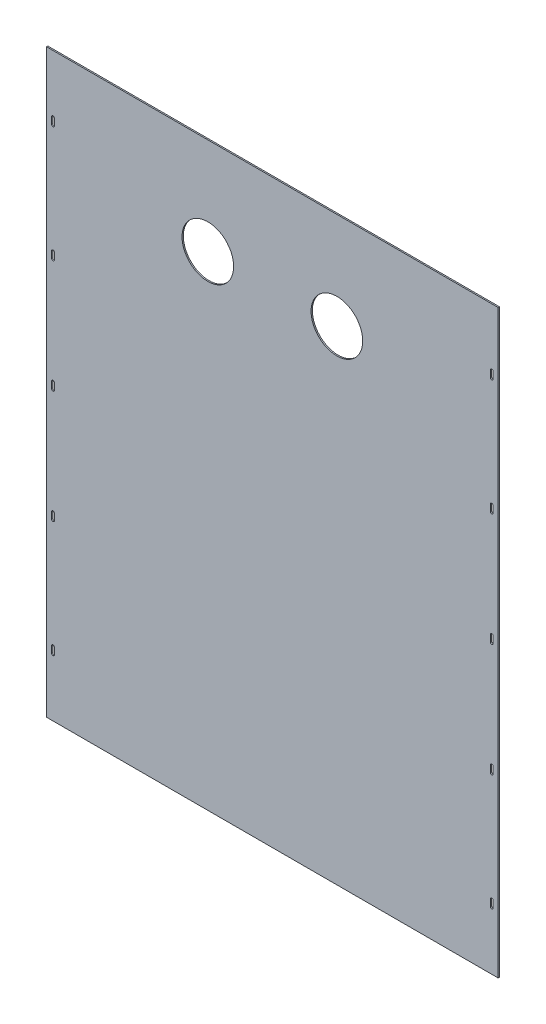
from build123d import *

# Parameters (mm, degrees)
SKETCH_1_W          = 700
SKETCH_1_H          = 900
EXTRUDE_1_DEPTH     = 2
CUT_EXTRUDE_1_DEPTH = 10
SKETCH_3_R          = 40
CUT_EXTRUDE_2_DEPTH = 10


with BuildPart() as part:
    # 草图1 → 凸台-拉伸1 (new body)
    with BuildSketch(Plane.XY):
        Rectangle(SKETCH_1_W, SKETCH_1_H)
    extrude(amount=EXTRUDE_1_DEPTH)

    # 草图2 → 切除-拉伸1 (cut)
    with BuildSketch(Plane.XY.offset(2)):
        with BuildLine():
            Line((-337.75, 180), (-337.75, 170))
            ThreePointArc((-337.75, 170), (-340, 167.75), (-342.25, 170))
            Line((-342.25, 170), (-342.25, 180))
            ThreePointArc((-342.25, 180), (-340, 182.25), (-337.75, 180))
        make_face()
        with BuildLine():
            Line((-342.25, -5), (-342.25, 5))
            ThreePointArc((-342.25, 5), (-340, 7.25), (-337.75, 5))
            Line((-337.75, 5), (-337.75, -5))
            ThreePointArc((-337.75, -5), (-340, -7.25), (-342.25, -5))
        make_face()
        with BuildLine():
            Line((337.75, 170), (337.75, 180))
            ThreePointArc((337.75, 180), (340, 182.25), (342.25, 180))
            Line((342.25, 180), (342.25, 170))
            ThreePointArc((342.25, 170), (340, 167.75), (337.75, 170))
        make_face()
        with BuildLine():
            Line((342.25, -5), (342.25, 5))
            ThreePointArc((342.25, 5), (340, 7.25), (337.75, 5))
            Line((337.75, 5), (337.75, -5))
            ThreePointArc((337.75, -5), (340, -7.25), (342.25, -5))
        make_face()
        with BuildLine():
            Line((-342.25, 360), (-342.25, 350))
            ThreePointArc((-342.25, 350), (-340, 347.75), (-337.75, 350))
            Line((-337.75, 350), (-337.75, 360))
            ThreePointArc((-337.75, 360), (-340, 362.25), (-342.25, 360))
        make_face()
        with BuildLine():
            Line((337.75, -170), (337.75, -180))
            ThreePointArc((337.75, -180), (340, -182.25), (342.25, -180))
            Line((342.25, -180), (342.25, -170))
            ThreePointArc((342.25, -170), (340, -167.75), (337.75, -170))
        make_face()
        with BuildLine():
            Line((342.25, 360), (342.25, 350))
            ThreePointArc((342.25, 350), (340, 347.75), (337.75, 350))
            Line((337.75, 350), (337.75, 360))
            ThreePointArc((337.75, 360), (340, 362.25), (342.25, 360))
        make_face()
        with BuildLine():
            Line((342.25, -360), (342.25, -350))
            ThreePointArc((342.25, -350), (340, -347.75), (337.75, -350))
            Line((337.75, -350), (337.75, -360))
            ThreePointArc((337.75, -360), (340, -362.25), (342.25, -360))
        make_face()
        with BuildLine():
            Line((-342.25, -360), (-342.25, -350))
            ThreePointArc((-342.25, -350), (-340, -347.75), (-337.75, -350))
            Line((-337.75, -350), (-337.75, -360))
            ThreePointArc((-337.75, -360), (-340, -362.25), (-342.25, -360))
        make_face()
        with BuildLine():
            Line((-337.75, -170), (-337.75, -180))
            ThreePointArc((-337.75, -180), (-340, -182.25), (-342.25, -180))
            Line((-342.25, -180), (-342.25, -170))
            ThreePointArc((-342.25, -170), (-340, -167.75), (-337.75, -170))
        make_face()
    extrude(amount=-CUT_EXTRUDE_1_DEPTH, mode=Mode.SUBTRACT)

    # 草图3 → 切除-拉伸2 (cut)
    with BuildSketch(Plane.XY.offset(2)):
        with Locations((-100, 300)):
            Circle(SKETCH_3_R)
        with Locations((100, 300)):
            Circle(SKETCH_3_R)
    extrude(amount=-CUT_EXTRUDE_2_DEPTH, mode=Mode.SUBTRACT)


solid = part.part
